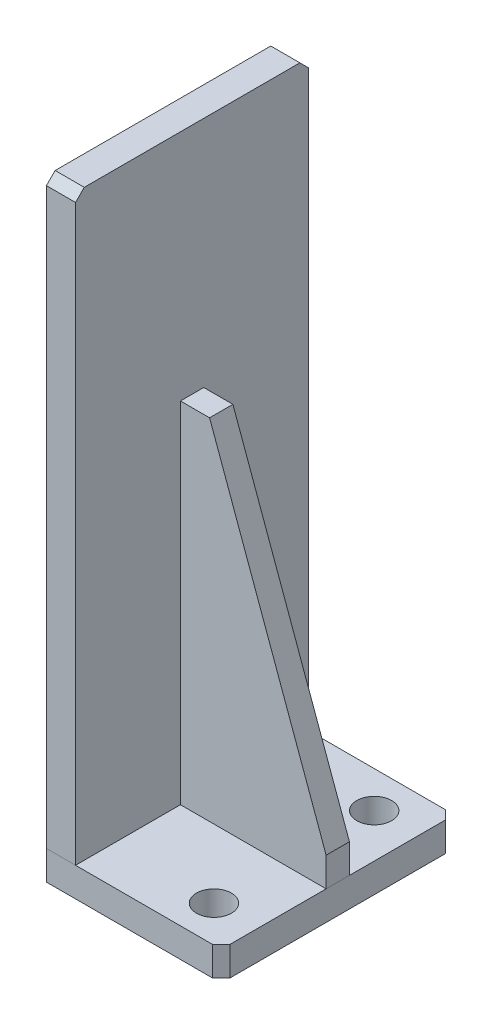
from build123d import *

# Parameters (mm, degrees)
SKETCH_1_W          = 60
SKETCH_1_H          = 80
EXTRUDE_1_DEPTH     = 5
SKETCH_2_W          = 10
SKETCH_2_H          = 80
EXTRUDE_2_DEPTH     = 200
CHAMFER_1_SIZE      = 3
CHAMFER_2_SIZE      = 3
EXTRUDE_3_DEPTH     = 4
SKETCH_7_R          = 6
CUT_EXTRUDE_1_DEPTH = 10


with BuildPart() as part:
    # 草图1 → 凸台-拉伸1 (new, symmetric)
    with BuildSketch(Plane(origin=(0, 0, 0), x_dir=(1, 0, 0), z_dir=(0, 1, 0))):
        Rectangle(SKETCH_1_W, SKETCH_1_H)
    extrude(amount=EXTRUDE_1_DEPTH, both=True)

    # 倒角1
    chamfer_1_edges = [part.edges().sort_by_distance(p)[0] for p in [
        (30, 0, 40),
        (30, 0, -40),
    ]]
    chamfer(chamfer_1_edges, length=CHAMFER_1_SIZE)

    # 草图7 → 切除-拉伸1 (cut)
    with BuildSketch(Plane(origin=(0, 5, 0), x_dir=(1, 0, 0), z_dir=(0, 1, 0))):
        with Locations(Location((15, -27.5, 0), (0, 0, 270))):
            Circle(SKETCH_7_R)
        with Locations(Location((15, 27.5, 0), (0, 0, 90))):
            Circle(SKETCH_7_R)
    extrude(amount=-CUT_EXTRUDE_1_DEPTH, mode=Mode.SUBTRACT)


with BuildPart() as body_2:
    # 草图2 → 凸台-拉伸2 (new body)
    with BuildSketch(Plane(origin=(0, 5, 0), x_dir=(1, 0, 0), z_dir=(0, 1, 0))):
        with Locations((-25, 0)):
            Rectangle(SKETCH_2_W, SKETCH_2_H)
    extrude(amount=EXTRUDE_2_DEPTH)

    # 倒角2
    chamfer_2_edges = [body_2.edges().sort_by_distance(p)[0] for p in [
        (-25, 205, -40),
        (-25, 205, 40),
    ]]
    chamfer(chamfer_2_edges, length=CHAMFER_2_SIZE)


with BuildPart() as body_3:
    # 草图6 → 凸台-拉伸3 (new, symmetric)
    with BuildSketch(Plane.XY):
        Polygon((-20, 125), (-10, 125), (30, 15), (30, 5), (-20, 5), align=None)
    extrude(amount=EXTRUDE_3_DEPTH, both=True)


solid = Compound([part.part, body_2.part, body_3.part])
